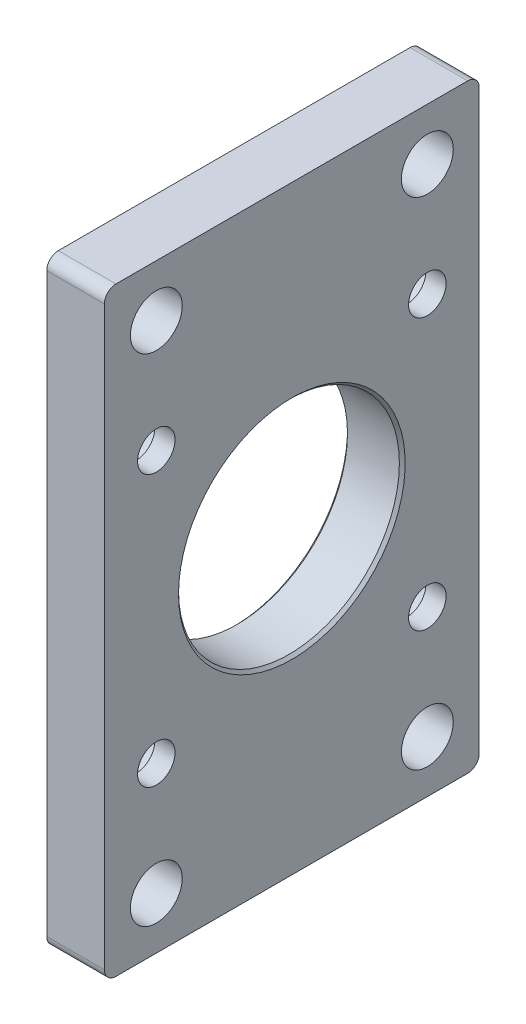
from build123d import *

# Parameters (mm, degrees)
BOSS_EXTRUDE1_DEPTH  = 10
LPATTERN1_COUNT      = 2
LPATTERN1_PITCH      = 47
LPATTERN1_COUNT_DIR2 = 2
LPATTERN1_PITCH_DIR2 = 47
LPATTERN2_COUNT      = 2
LPATTERN2_PITCH      = 47
LPATTERN2_COUNT_DIR2 = 2
LPATTERN2_PITCH_DIR2 = 86


with BuildPart() as part:
    # Sketch1 → Boss-Extrude1 (new body)
    with BuildSketch(Plane(origin=(0, 0, 0), x_dir=(0, 0, -1), z_dir=(1, 0, 0))):
        with BuildLine():
            Line((-30.5, -52), (30.5, -52))
            ThreePointArc((30.5, -52), (31.914213562, -51.414213562), (32.5, -50))
            Line((32.5, -50), (32.5, 50))
            ThreePointArc((32.5, 50), (31.914213562, 51.414213562), (30.5, 52))
            Line((30.5, 52), (-30.5, 52))
            ThreePointArc((-30.5, 52), (-31.914213562, 51.414213562), (-32.5, 50))
            Line((-32.5, 50), (-32.5, -50))
            ThreePointArc((-32.5, -50), (-31.914213562, -51.414213562), (-30.5, -52))
        make_face()
    extrude(amount=BOSS_EXTRUDE1_DEPTH)

    # Sketch2 → Cut-Revolve1 (revolve, cut)
    with BuildSketch(Plane(origin=(0, 0, 0), x_dir=(1, 0, 0), z_dir=(0, 1, 0))):
        Polygon((10, 0), (10, -19.65), (9.5, -19.15), (0.5, -19.15), (0, -19.65), (0, 0), align=None)
    revolve(axis=Axis((0, 0, 0), (1, 0, 0)), mode=Mode.SUBTRACT)

    # Sketch3 → Cut-Revolve2 (revolve, cut)
    with BuildSketch(Plane(origin=(0, -23.5, 0), x_dir=(1, 0, 0), z_dir=(0, 1, 0))):
        Polygon((10, 23.5), (10, 20.25), (6.5, 20.25), (6.5, 18.25), (0.5, 18.25), (0, 17.75), (0, 23.5), align=None)
    cut_revolve2 = revolve(axis=Axis((0, -23.5, -23.5), (1, 0, 0)), mode=Mode.SUBTRACT)

    # LPattern1: Cut-Revolve2 2 × 2
    with Locations(*[(0, i * LPATTERN1_PITCH, j * LPATTERN1_PITCH_DIR2) for i in range(LPATTERN1_COUNT) for j in range(LPATTERN1_COUNT_DIR2) if (i, j) != (0, 0)]):
        add(cut_revolve2, mode=Mode.SUBTRACT)

    # Sketch5 → Cut-Revolve3 (revolve, cut)
    with BuildSketch(Plane(origin=(0, -43, 0), x_dir=(1, 0, 0), z_dir=(0, 1, 0))):
        Polygon((0, -23.5), (0, -18.5), (0.5, -19), (10, -19), (10, -23.5), align=None)
    cut_revolve3 = revolve(axis=Axis((10, -43, 23.5), (-1, 0, 0)), mode=Mode.SUBTRACT)

    # LPattern2: Cut-Revolve3 2 × 2
    with Locations(*[(0, j * LPATTERN2_PITCH_DIR2, -i * LPATTERN2_PITCH) for i in range(LPATTERN2_COUNT) for j in range(LPATTERN2_COUNT_DIR2) if (i, j) != (0, 0)]):
        add(cut_revolve3, mode=Mode.SUBTRACT)


solid = part.part
